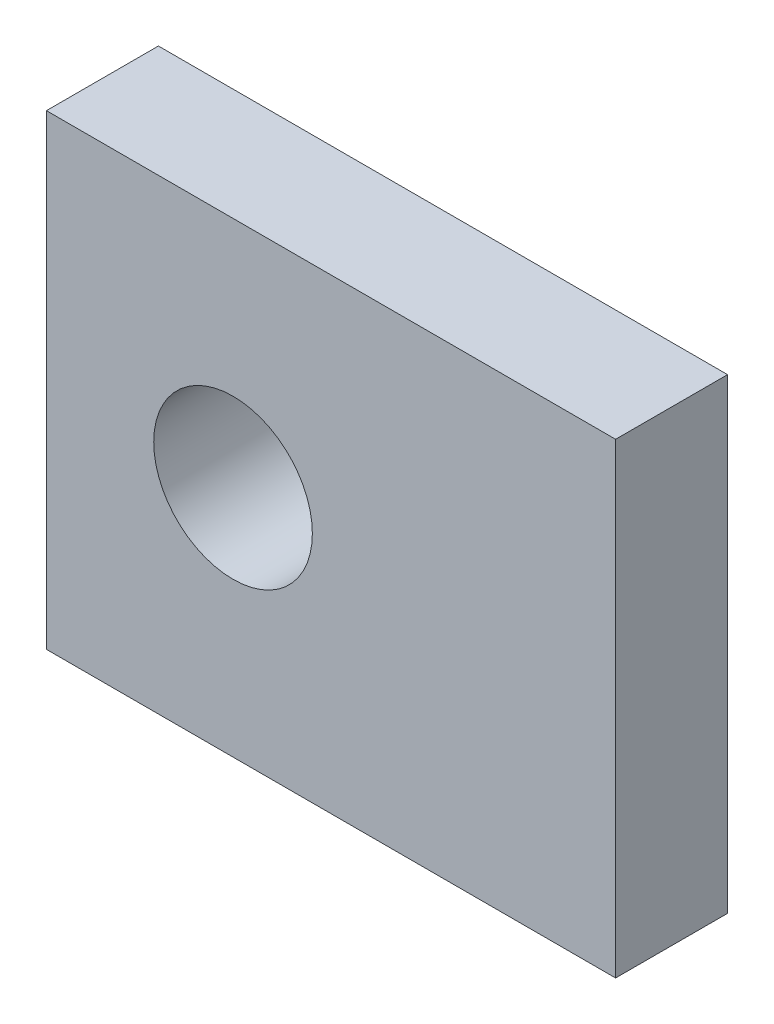
from build123d import *

# Parameters (mm, degrees)
SKETCH1_W           = 30.5
SKETCH1_H           = 25
SKETCH1_R           = 4.25
BOSS_EXTRUDE1_DEPTH = 6


with BuildPart() as part:
    # Sketch1 → Boss-Extrude1 (new body)
    with BuildSketch(Plane.XY):
        with Locations((-21.35, -55.605666667)):
            Rectangle(SKETCH1_W, SKETCH1_H)
        with Locations((-26.6, -55.605666667)):
            Circle(SKETCH1_R, mode=Mode.SUBTRACT)
    extrude(amount=BOSS_EXTRUDE1_DEPTH)


solid = part.part
